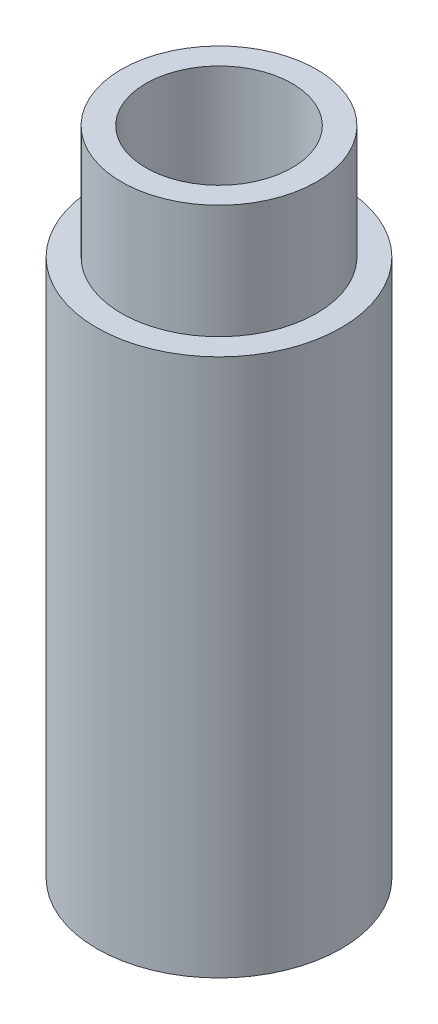
from build123d import *


with BuildPart() as part:
    # Sketch2 → Revolve1 (revolve)
    with BuildSketch(Plane.XY):
        Polygon((51.067350004, -25.488807327), (51.067350004, 80.061192673), (56.117350004, 80.061192673), (56.117350004, 107.791192673), (51.117350004, 107.791192673), (51.117350004, 97.791192673), (51.117350004, 84.511192673), (46.067350004, 84.511192673), (46.067350004, -25.488807327), align=None)
    revolve(axis=Axis((71.067350004, 101.177656429, 0), (0, -1, 0)))


solid = part.part
